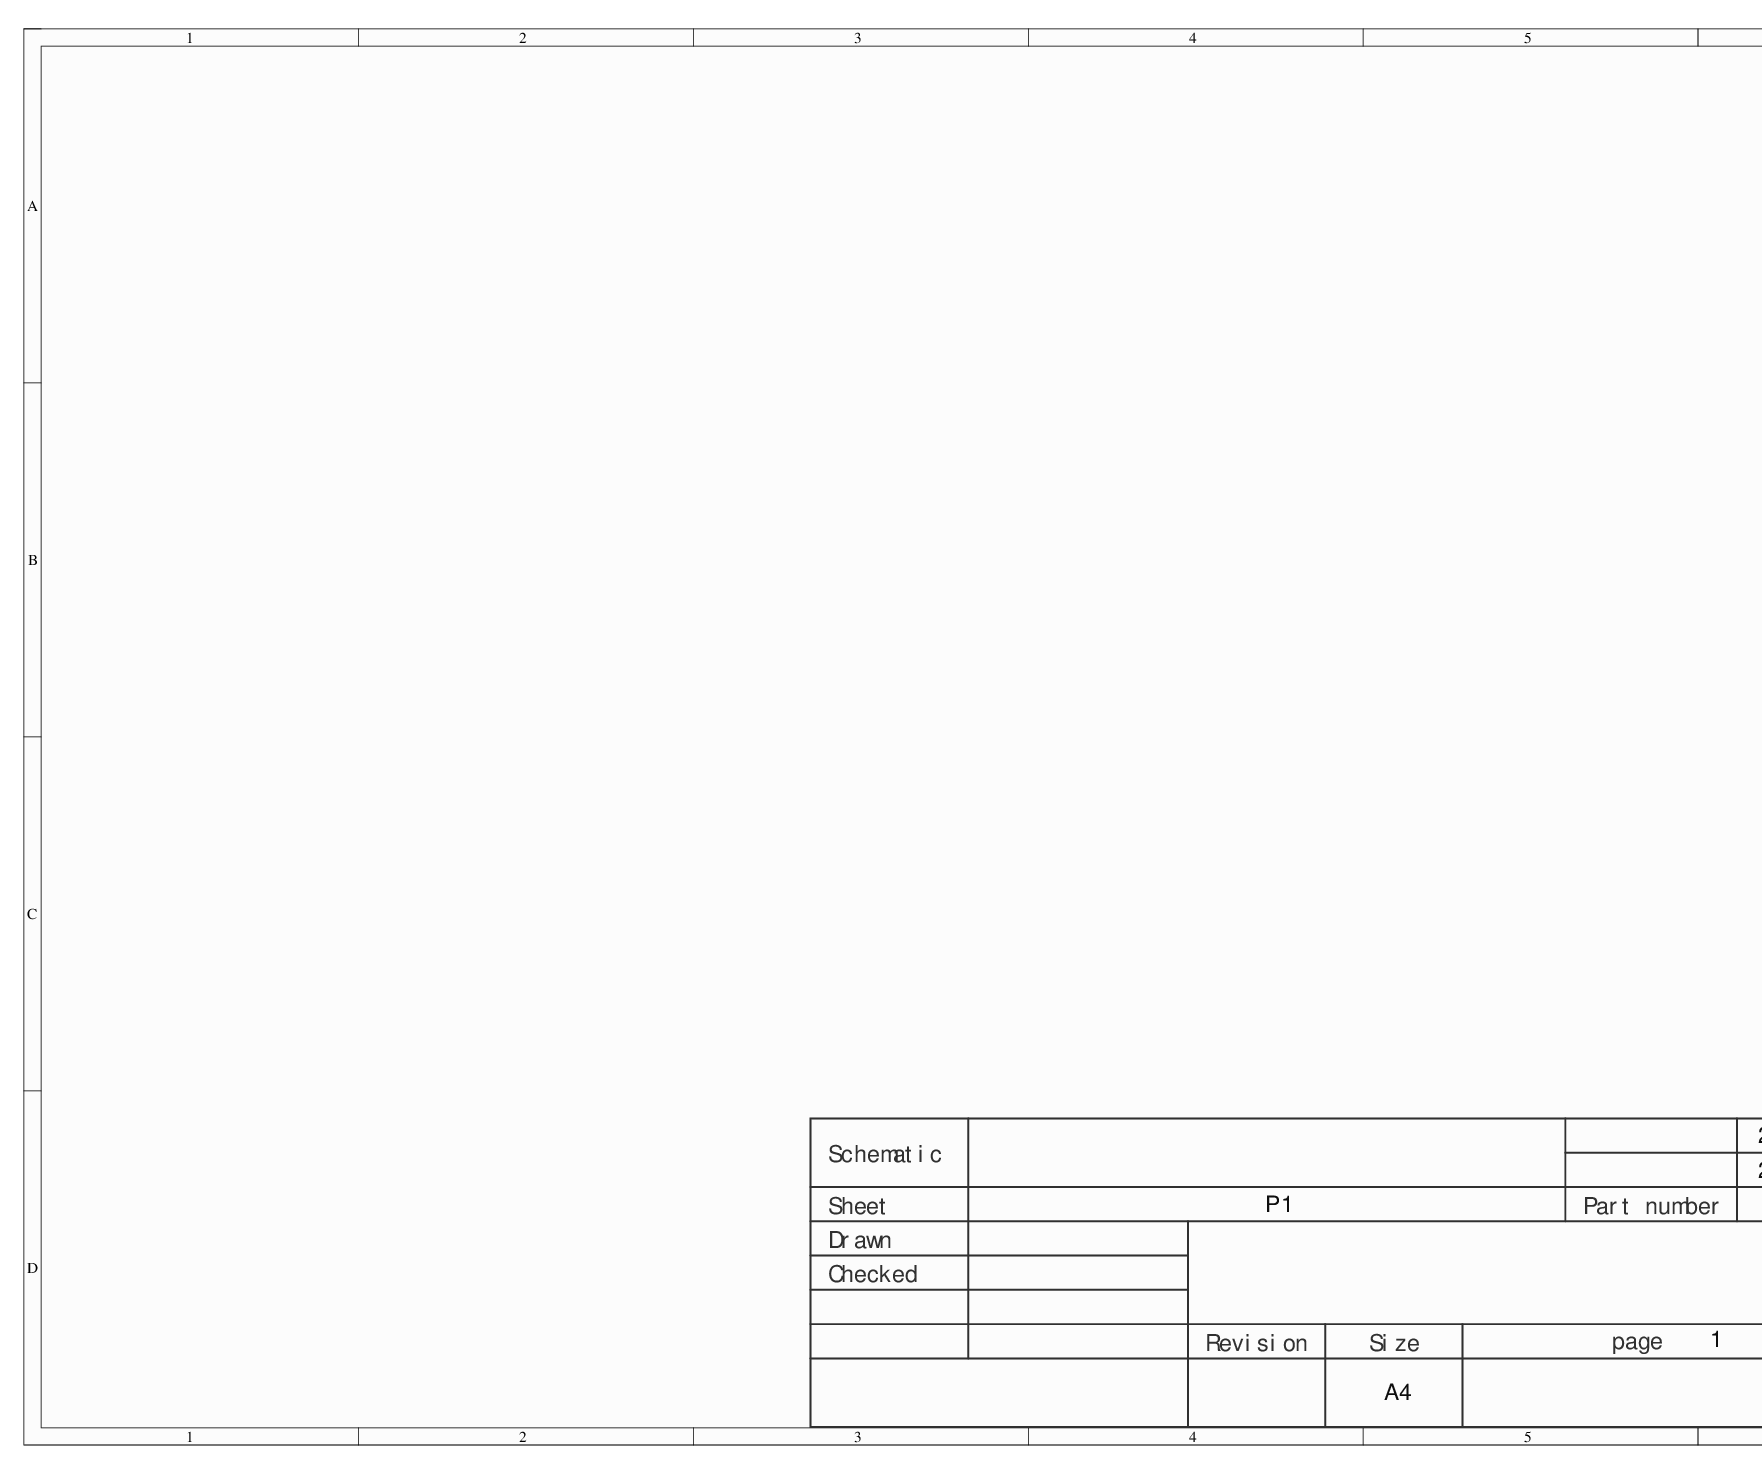
[diagram p0: MISC82093-2.schdoc, top left]
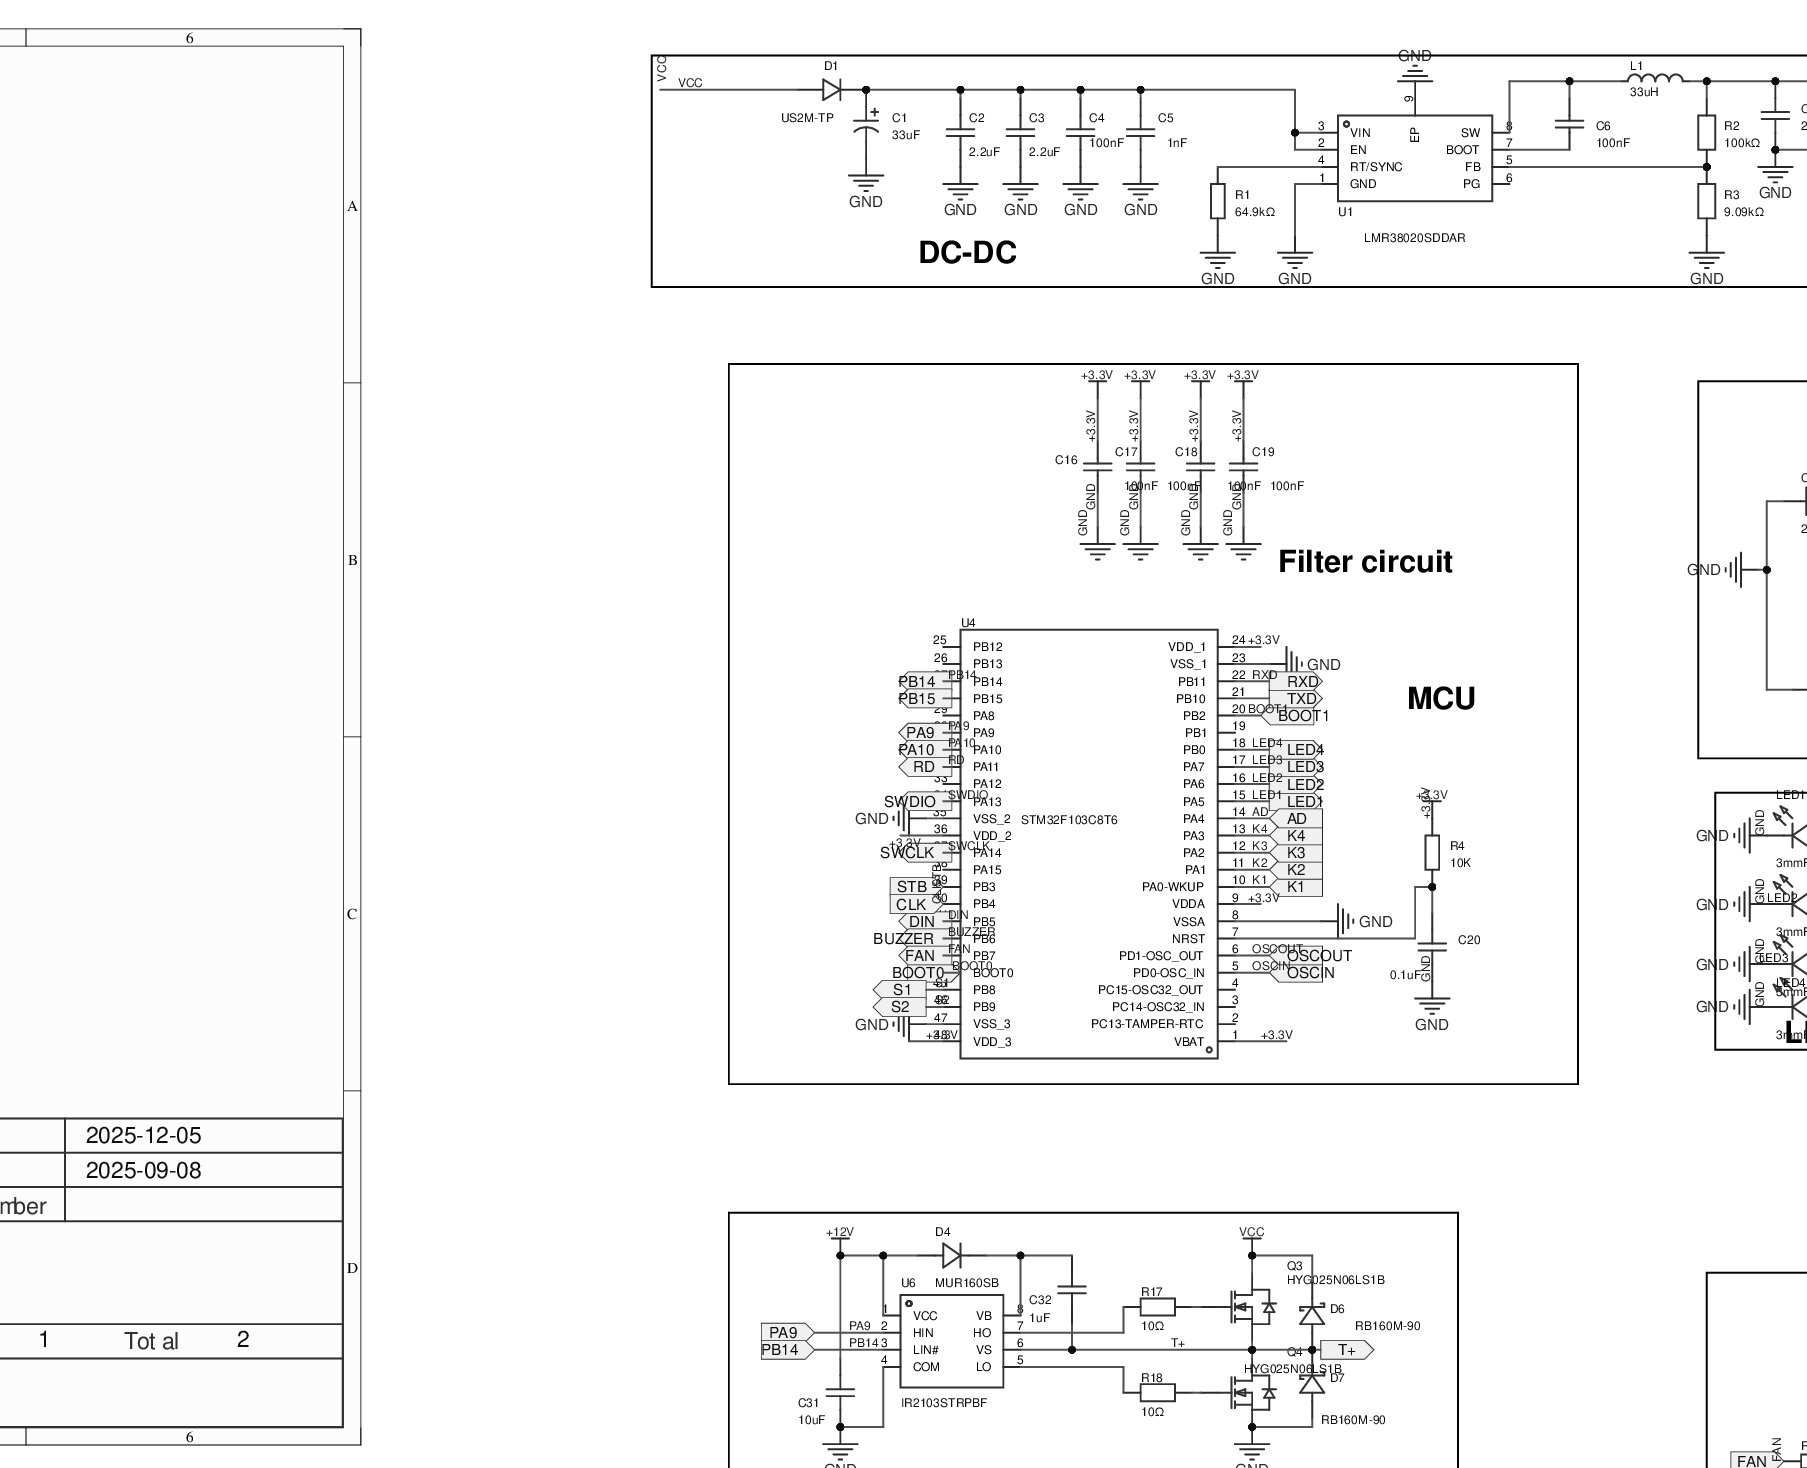
[diagram p1: MISC82093-2.schdoc, top middle]
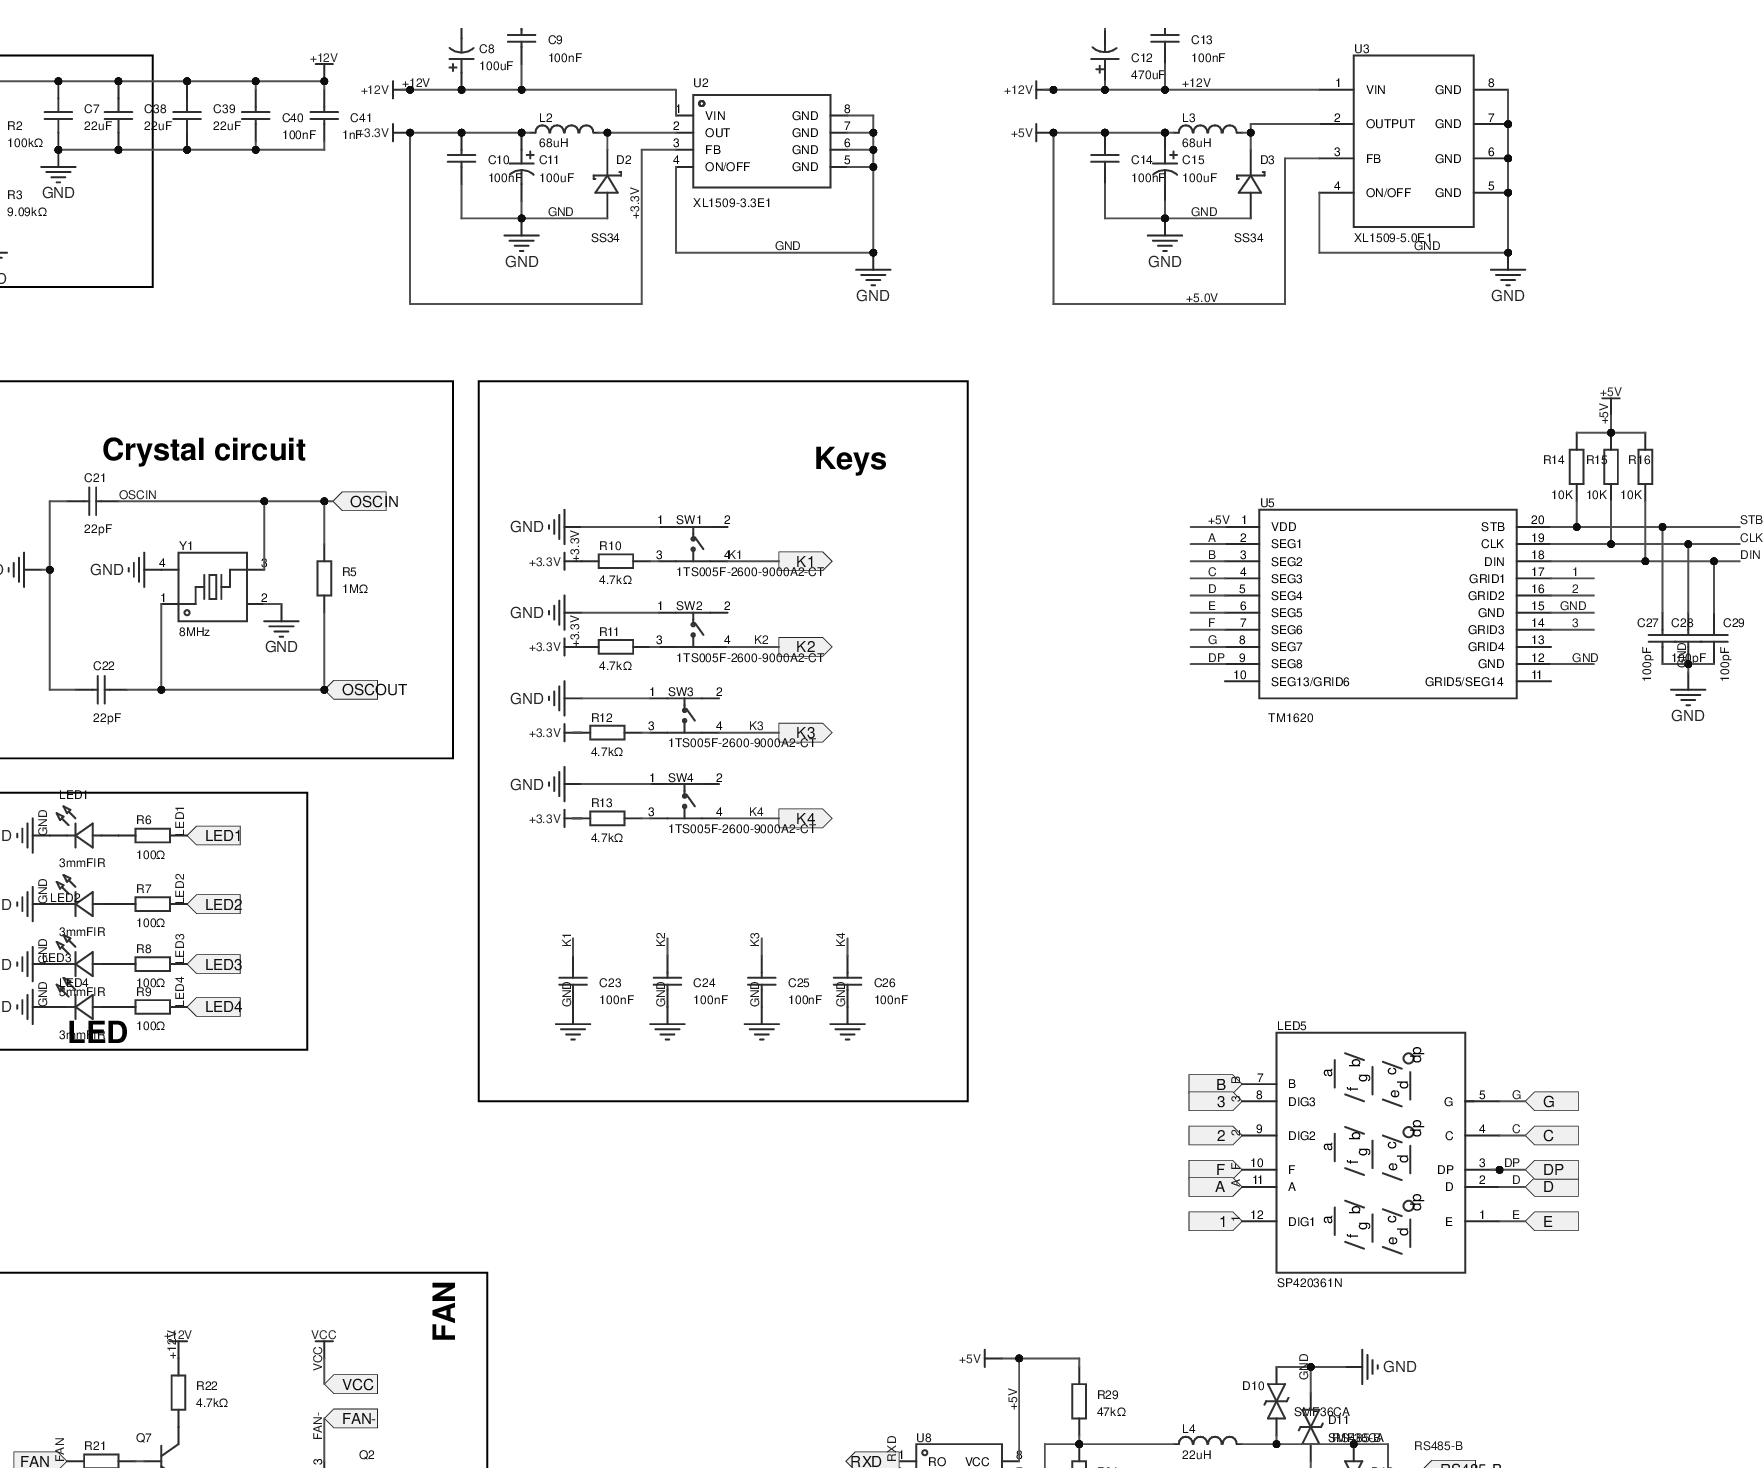
[diagram p2: MISC82093-2.schdoc, top right]
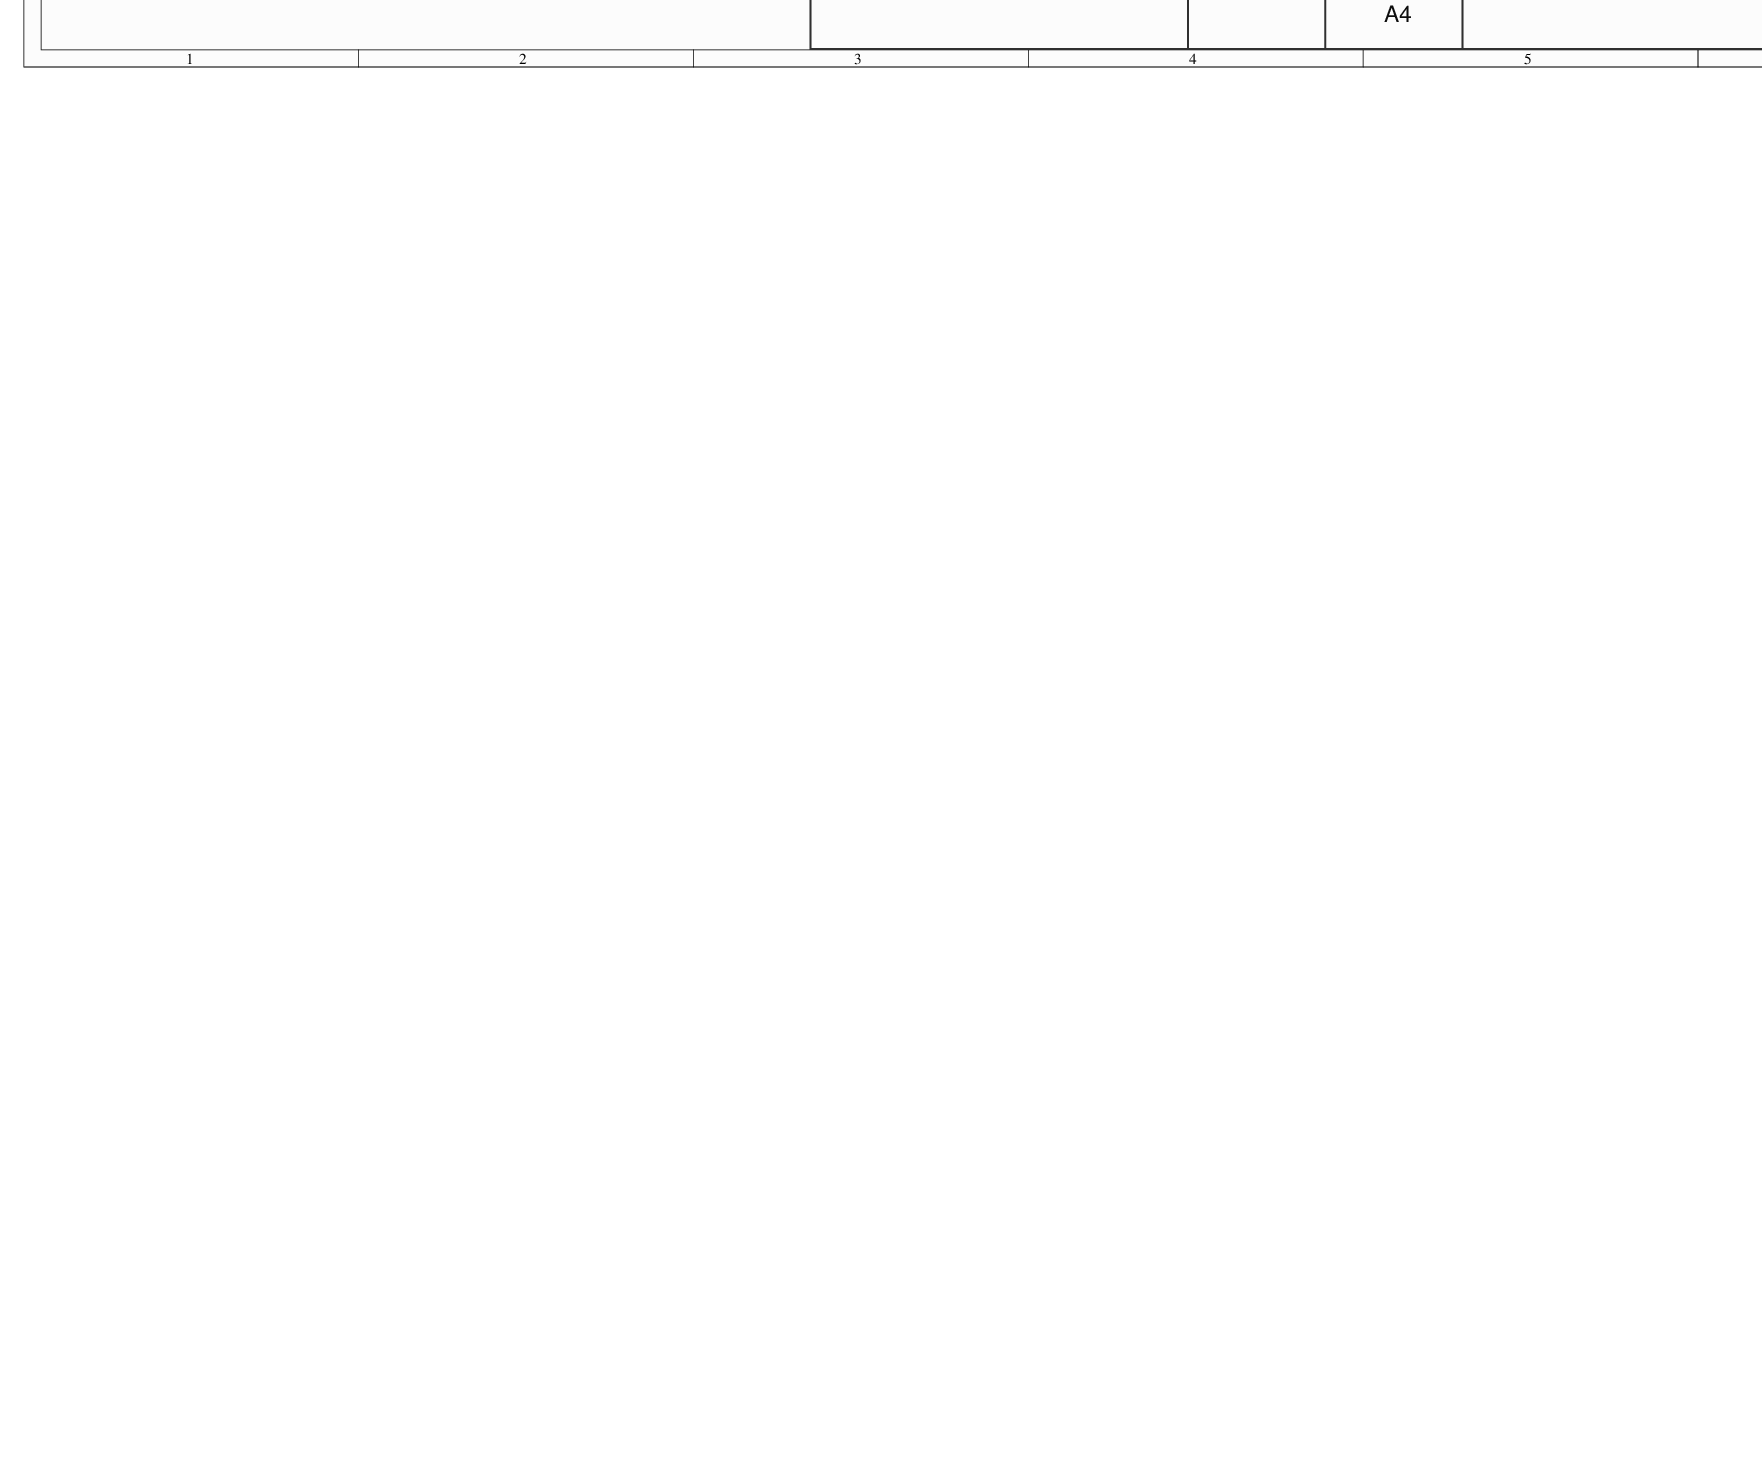
[diagram p3: MISC82093-2.schdoc, bottom left]
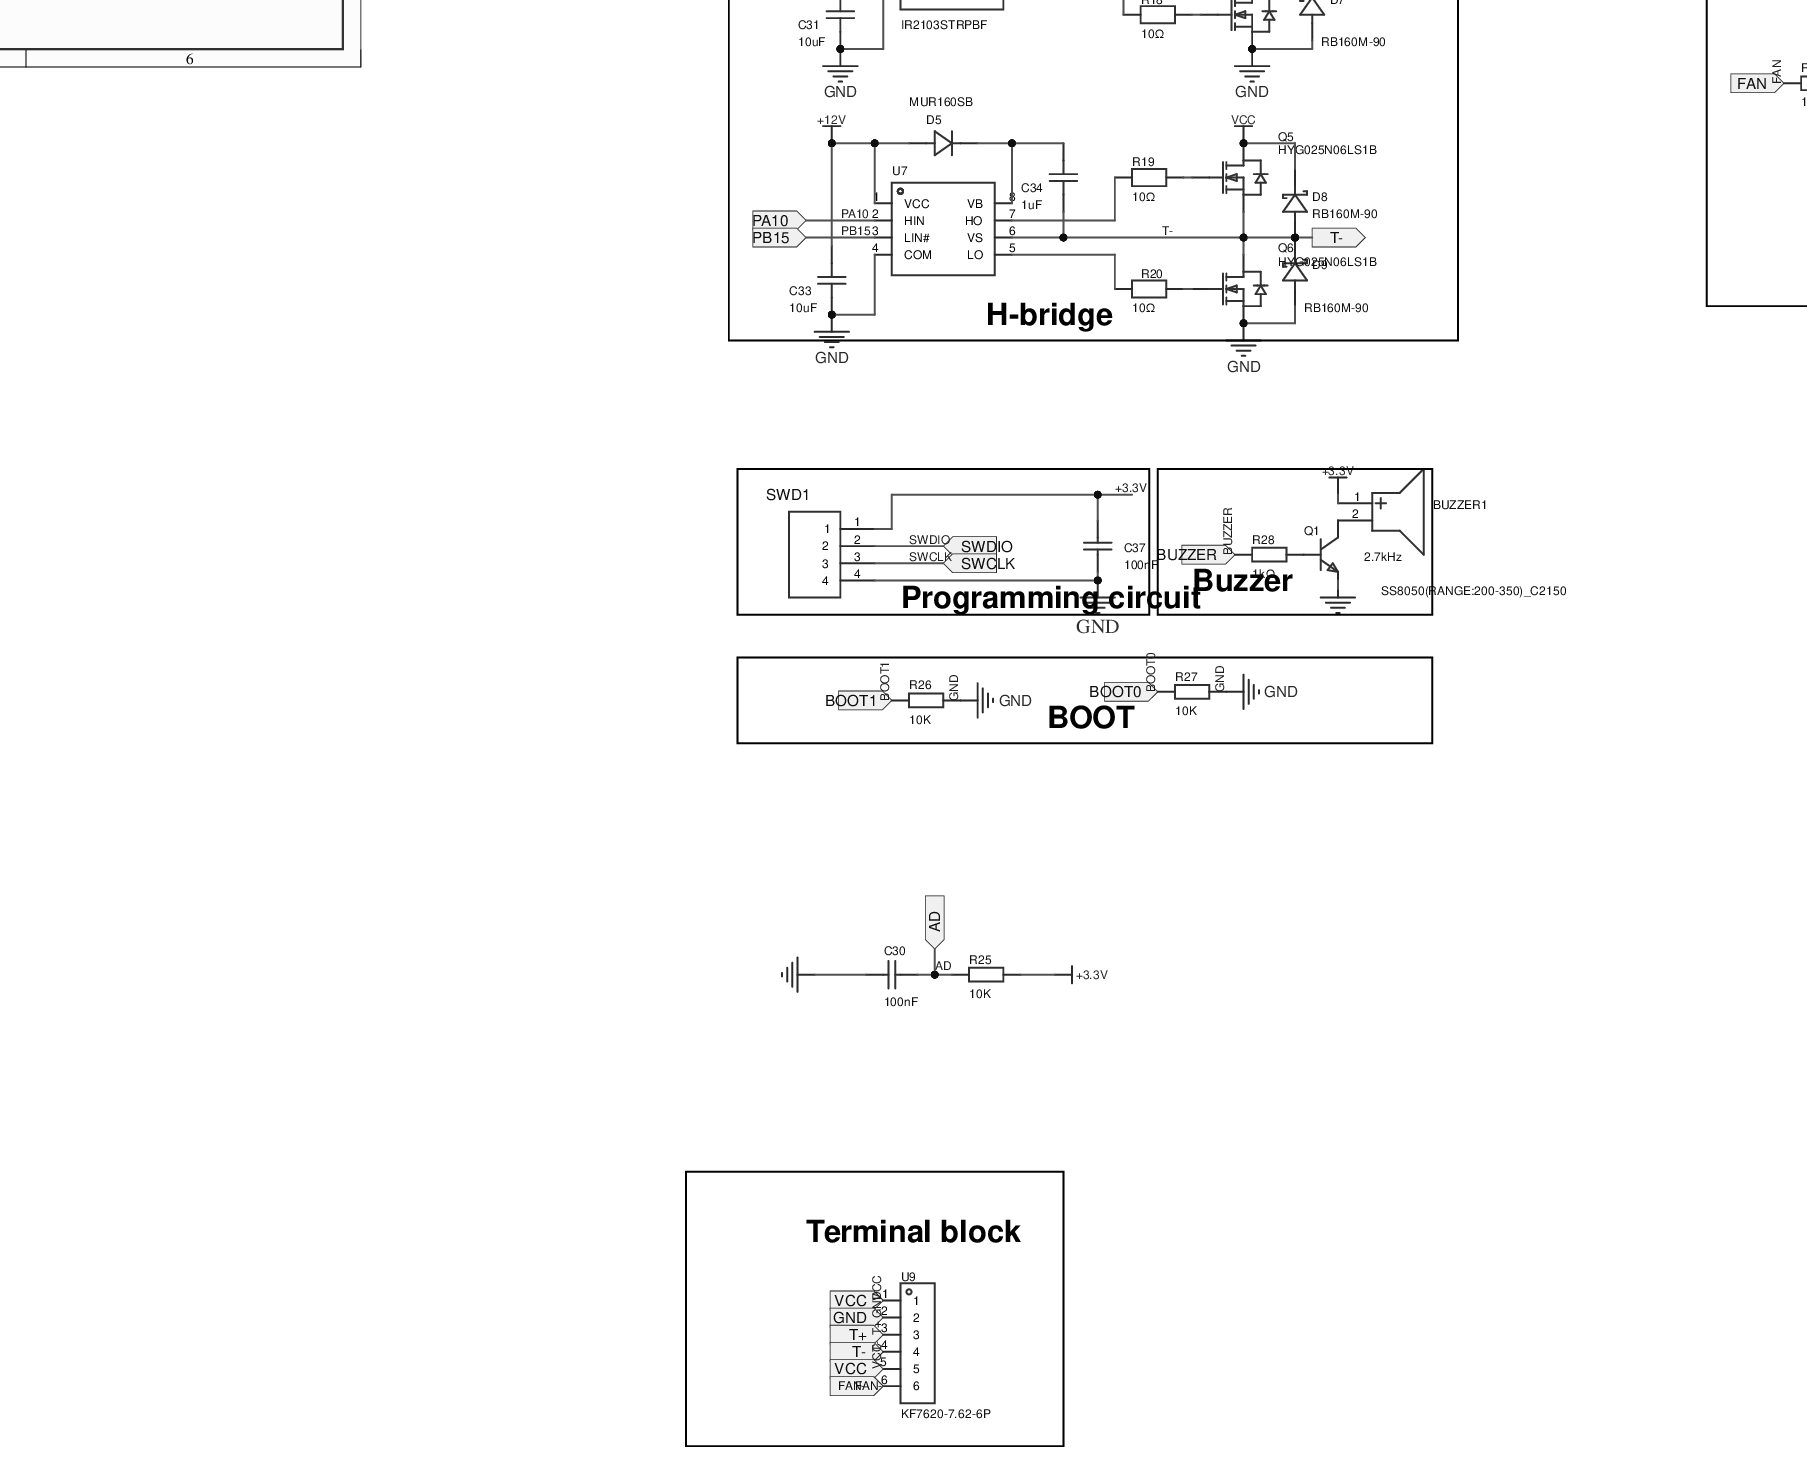
[diagram p4: MISC82093-2.schdoc, bottom middle]
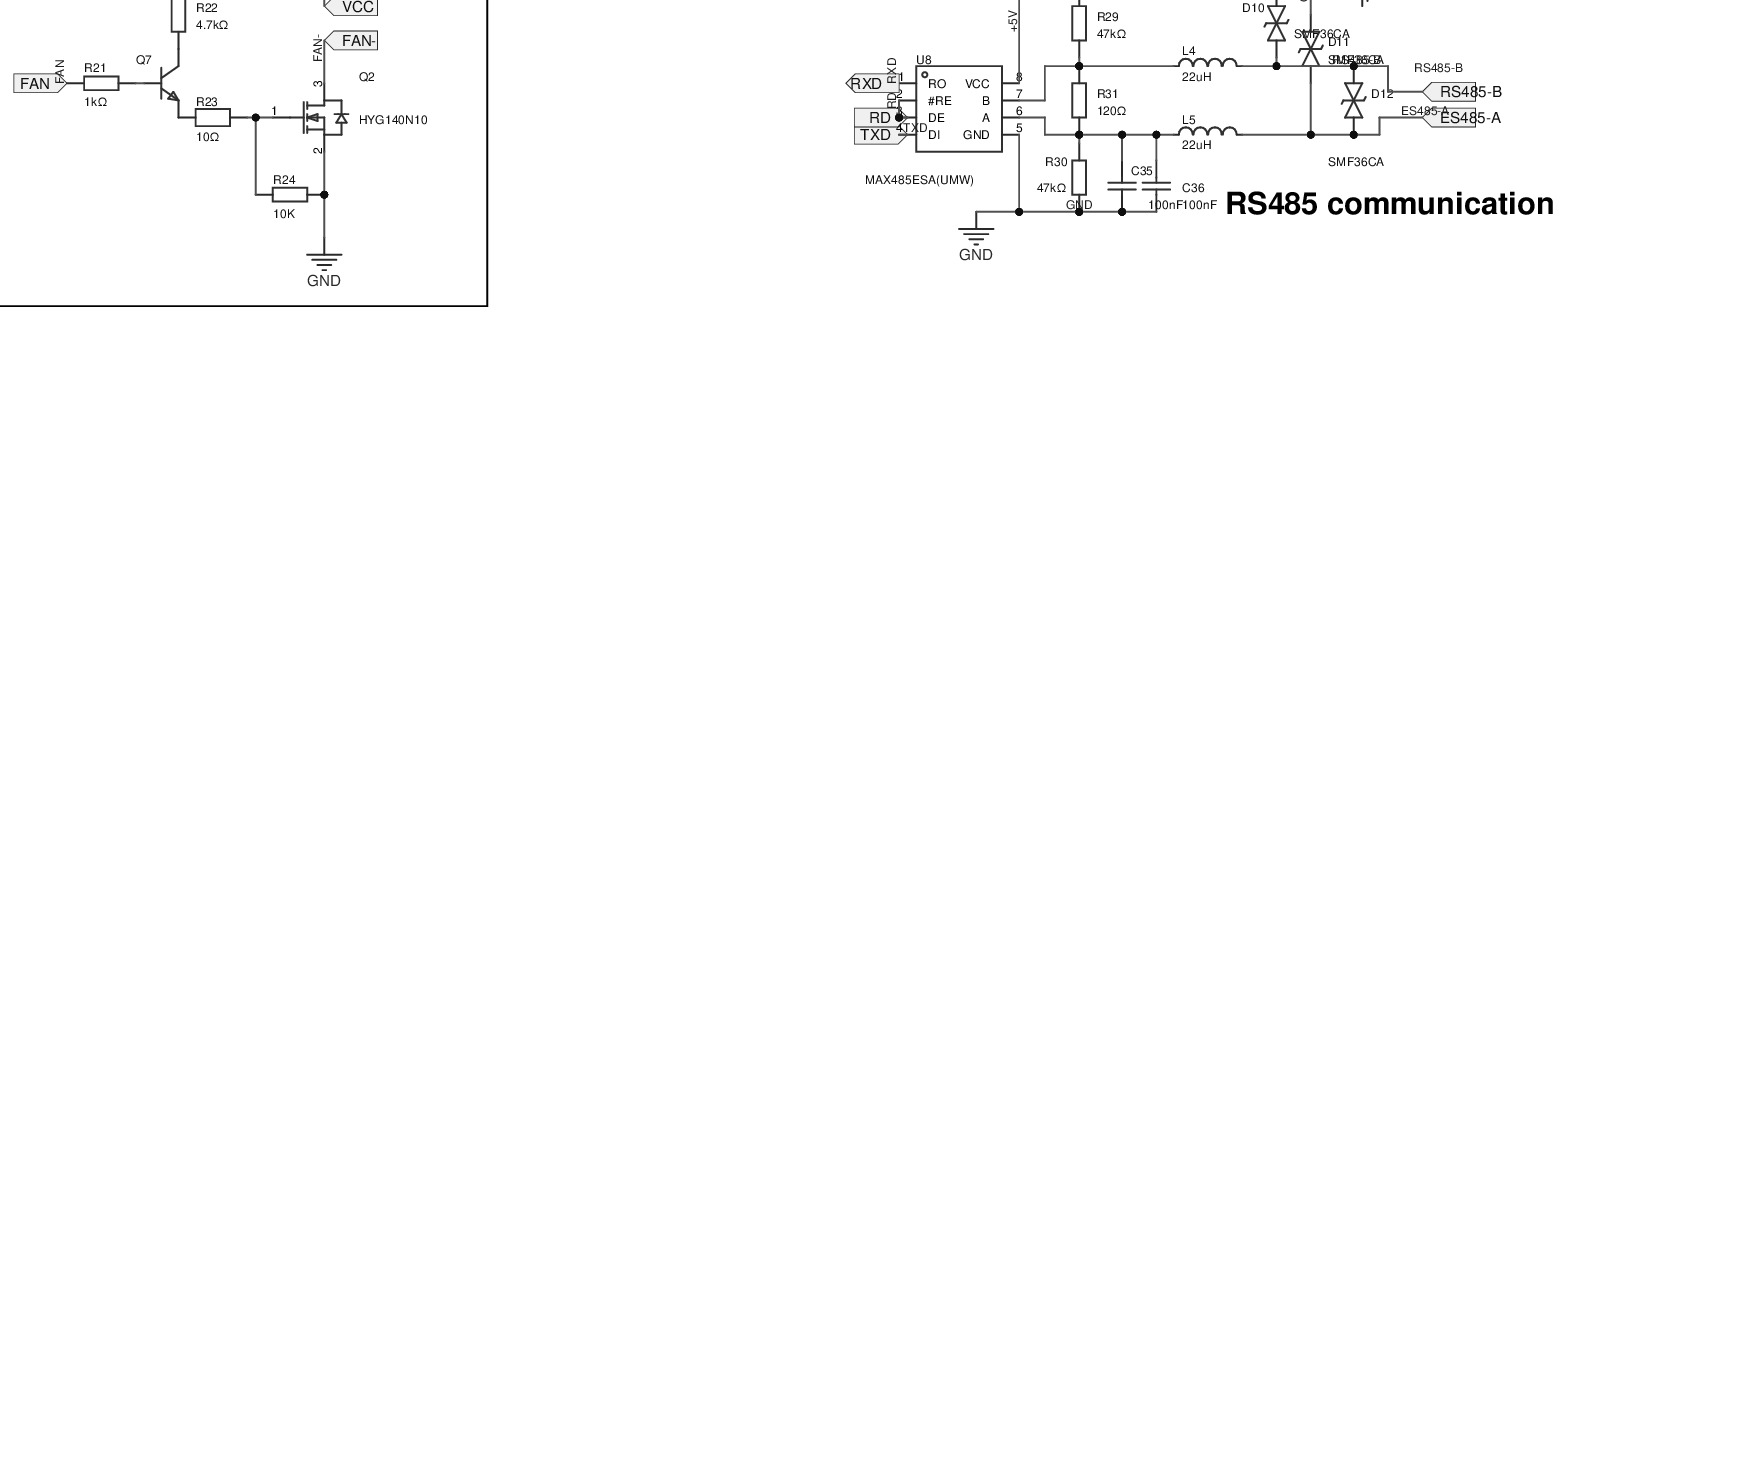
[diagram p5: MISC82093-2.schdoc, bottom right]
# Altium schematic sheet MISC82093-2.schdoc (part 1 of 2)
size 297 x 209 mm; Version: V1.0; @Project Name: MISC82093; @Page Count: 2; @Update Date: 2025-12-05; @Create Date: 2025-09-08; @Schematic Name: MISC82093; @Page No: 1; @Board Name: MISC82093; @Create Time: 16:21:40; @Update Time: 16:58:32

## Parts
BUZZER1  2.7kHz  [BUZ-SMD_L9.6-W9.6-LS10.0-R]
C1  33uF  [CAP-TH_BD8.0-P3.50-D1.0-FD]
C2  2.2uF  [C1206]
C3  2.2uF  [C1206]
C4  100nF  [C1206]
C5  1nF  [C1206]
C6  100nF  [C0805]
C7  22uF  [C1210]
C8  100uF  [CAP-SMD_BD6.3-L6.6-W6.6-LS7.3-FD_JVS25V100M6X4]
C9  100nF  [C0805]
C10  100nF  [C0805]
C11  100uF  [CAP-SMD_BD6.3-L6.6-W6.6-LS7.3-FD_JVS25V100M6X4]
C12  470uF  [CAP-TH_BD10.0-P5.00-D1.0-FD]
C13  100nF  [C0805]
C14  100nF  [C0805]
C15  100uF  [CAP-SMD_BD6.3-L6.6-W6.6-LS7.3-FD_JVS25V100M6X4]
C16  100nF  [C0805]
C17  100nF  [C0805]
C18  100nF  [C0805]
C19  100nF  [C0805]
C20  0.1uF  [C0805]
C21  22pF  [C0805]
C22  22pF  [C0805]
C23  100nF  [C0805]
C24  100nF  [C0805]
C25  100nF  [C0805]
C26  100nF  [C0805]
C27  100pF  [C0805]
C28  100pF  [C0805]
C29  100pF  [C0805]
C30  100nF  [C0805]
C31  10uF  [C0805]
C32  1uF  [C0805]
C33  10uF  [C0805]
C34  1uF  [C0805]
C35  100nF  [C0805]
C36  100nF  [C0805]
C37  100nF  [C0805]
C38  22uF  [C1210]
C39  22uF  [C1210]
C40  100nF  [C0805]
C41  1nF  [C0805]
D1  US2M-TP  [SMB_L4.6-W3.6-LS5.3-RD]
D2  SS34  [SMA_L4.3-W2.6-LS5.2-RD]
D3  SS34  [SMA_L4.3-W2.6-LS5.2-RD]
D4  MUR160SB  [SMB_L4.6-W3.6-LS5.3-RD]
D5  MUR160SB  [SMB_L4.6-W3.6-LS5.3-RD]
D6  RB160M-90  [SOD-123FL_L2.7-W1.8-LS3.7-RD]
D7  RB160M-90  [SOD-123FL_L2.7-W1.8-LS3.7-RD]
D8  RB160M-90  [SOD-123FL_L2.7-W1.8-LS3.7-RD]
D9  RB160M-90  [SOD-123FL_L2.7-W1.8-LS3.7-RD]
D10  SMF36CA  [SOD-123_L2.7-W1.8-LS3.7-BI]
D11  SMF36CA  [SOD-123_L2.7-W1.8-LS3.7-BI]
D12  SMF36CA  [SOD-123_L2.7-W1.8-LS3.7-BI]
L1  33uH  [IND-SMD_L11.5-W10.0_FXL1040]
L2  68uH  [IND-SMD_L7.1-W6.6_H5.0]
L3  68uH  [IND-SMD_L7.1-W6.6_H5.0]
L4  22uH  [L1206]
L5  22uH  [L1206]
LED1  3mmFIR  [LED-TH_BD3.0-P2.54-FD]
LED2  3mmFIR  [LED-TH_BD3.0-P2.54-FD]
LED3  3mmFIR  [LED-TH_BD3.0-P2.54-FD]
LED4  3mmFIR  [LED-TH_BD3.0-P2.54-FD]
LED5  SP420361N  [LED-SEG-TH_SP420361N]
Q1  SS8050(RANGE:200-350)  [SOT-23-3_L2.9-W1.3-P1.90-LS2.4-BR]  (value not drawn)
Q2  HYG140N10  [TO-252-3_L6.6-W6.1-P4.58-LS10.1-BR]
Q3  HYG025N06LS1B  [TO-263-2_L10.2-W8.7-P5.08-LS15.1-BR]
Q4  HYG025N06LS1B  [TO-263-2_L10.2-W8.7-P5.08-LS15.1-BR]
Q5  HYG025N06LS1B  [TO-263-2_L10.2-W8.7-P5.08-LS15.1-BR]
Q6  HYG025N06LS1B  [TO-263-2_L10.2-W8.7-P5.08-LS15.1-BR]
Q7  SS8050(RANGE:200-350)  [SOT-23-3_L2.9-W1.3-P1.90-LS2.4-BR]  (value not drawn)
R1  64.9kΩ  [R0805]
R2  100kΩ  [R0805]
R3  9.09kΩ  [R0805]
R4  10K  [R0805]
R5  1MΩ  [R0805]
R6  100Ω  [R0805]
R7  100Ω  [R0805]
R8  100Ω  [R0805]
R9  100Ω  [R0805]
R10  4.7kΩ  [R0805]
R11  4.7kΩ  [R0805]
R12  4.7kΩ  [R0805]
R13  4.7kΩ  [R0805]
R14  10K  [R0805]
R15  10K  [R0805]
R16  10K  [R0805]
R17  10Ω  [R0805]
R18  10Ω  [R0805]
R19  10Ω  [R0805]
R20  10Ω  [R0805]
R21  1kΩ  [R0805]
R22  4.7kΩ  [R0805]
R23  10Ω  [R0805]
R24  10K  [R0805]
R25  10K  [R0805]
R26  10K  [R0805]
R27  10K  [R0805]
R28  1kΩ  [R0805]
R29  47kΩ  [R0805]
R30  47kΩ  [R0805]
R31  120Ω  [R0805]
SW1  1TS005F-2600-9000A2-CT  [SW-SMD_4P-L6.0-W6.0-P4.50-LS9.0-2]
SW2  1TS005F-2600-9000A2-CT  [SW-SMD_4P-L6.0-W6.0-P4.50-LS9.0-2]
SW3  1TS005F-2600-9000A2-CT  [SW-SMD_4P-L6.0-W6.0-P4.50-LS9.0-2]
SW4  1TS005F-2600-9000A2-CT  [SW-SMD_4P-L6.0-W6.0-P4.50-LS9.0-2]
SWD1  220S-1*4P H=8.5MM Ytype Gold-plated  [DIP-1X4P2.54]  (value not drawn)
U1  LMR38020SDDAR  [ESOP-8_L4.9-W3.9-P1.27-LS6.0-BL-EP-1]
U2  XL1509-3.3E1  [SOP-8_L4.9-W3.9-P1.27-LS6.0-BL]
U3  XL1509-5.0E1  [SOIC-8_L5.0-W4.0-P1.27-LS6.0-BL]
U4  STM32F103C8T6  [LQFP-48_L7.0-W7.0-P0.50-LS9.0-BL]
U5  TM1620  [SOIC-20_L13.0-W7.6-P1.27-LS10.3-BL]
U6  IR2103STRPBF  [SOIC-8_L4.9-W3.9-P1.27-LS6.0-BL]
U7  (no value)  [SOIC-8_L4.9-W3.9-P1.27-LS6.0-BL]
U8  MAX485ESA(UMW)  [SOP-8_L5.0-W4.0-P1.27-LS6.0-BL]
U9  KF7620-7.62-6P  [CONN-TH_6P-P7.62_KF7620-7.62-6P]
Y1  8MHz  [CRYSTAL-SMD_4P-L3.2-W2.5-BL]

## Blocks framed on the sheet
DC-DC: C1-C7 C38 D1 L1 R1-R3 U1
Crystal circuit: C21 C22 R5 Y1
Keys: C23-C26 R10-R13 SW1-SW4
LED: LED1-LED4 R6-R9
H-bridge: C31-C34 D4-D9 Q3-Q6 R17-R20 U6 U7
FAN: Q2 Q7 R21-R24
Programming circuit: C37 SWD1
Buzzer: BUZZER1 Q1 R28
BOOT: R26 R27
Terminal block: U9

## Ports
1 (in), 2 (in), 3 (in), A (in), AD (in), B (in), BOOT0 (in), BOOT1 (in), BUZZER (in), BUZZER (out), C (in), CLK (in), D (in), DIN (out), DP (in), E (in), ES485-A (in), F (in), FAN (in), FAN (out), FAN- (in), G (in), GND (in), K1 (in), K1 (out), K2 (in), K2 (out), K3 (in), K3 (out), K4 (in), K4 (out), LED1 (in), LED1 (out), LED2 (in), LED2 (out), LED3 (in), LED3 (out), LED4 (in), LED4 (out), OSCIN (in), OSCOUT (in), PA9 (in), PA9 (out), PA10 (in), PA10 (out), PB14 (in), PB14 (out), PB15 (in), PB15 (out), RD (in), RD (out), RS485-B (in), RXD (out), S1 (out), S2 (out), STB (in), SWCLK (in), SWCLK (out), SWDIO (in), SWDIO (out), T+ (in), T+ (out), T- (in), T- (out), TXD (in), TXD (out), VCC (in)

## Nets
+3.3V: BUZZER1.1(+) C10.2 C11.1 C16.2 C17.2 C18.2 C19.2 C37.2 L2.1 R4.2 R10.1 R11.1 R12.1 R13.1 R25.2 SWD1.1 U2.3(FB) U4.1(VBAT) U4.9(VDDA) U4.24(VDD_1) U4.36(VDD_2) U4.48(VDD_3)
+5.0V: C14.2 C15.1 L3.1 R14.2 R15.2 R16.2 R29.2 U3.3(FB) U5.1(VDD) U8.8(VCC)  [also labelled +5V]
+12V: C7.2 C8.1 C9.1 C12.1 C13.1 C31.2 C33.2 C38.2 C39.2 C40.2 C41.2 D4.2(A) D5.2(A) L1.2 R2.2 R22.2 U2.1(VIN) U3.1(VIN) U6.1(VCC) U7.1(VCC)
GND: C1.2 C2.1 C3.1 C4.1 C5.1 C7.1 C8.2 C9.2 C10.1 C11.2 C12.2 C13.2 C14.1 C15.2 C16.1 C17.1 C18.1 C19.1 C20.1 C21.2 C22.2 C23.1 C24.1 C25.1 C26.1 C27.2 C28.2 C29.1 C30.2 C31.1 C33.1 C35.1 C36.2 C37.1 C38.1 C39.1 C40.1 C41.1 D2.2(A) D3.2(A) D7.2(+) D9.2(+) D10.2 D11.2 LED1.2(K) LED2.2(K) LED3.2(K) LED4.2(K) Q1.2(E) Q2.2(S) Q4.3(S) Q6.3(S) R1.1 R3.1 R24.2 R26.2 R27.2 R30.1 SW1.1 SW2.1 SW3.1 SW4.1 SWD1.4 U1.1(GND) U1.9(EP) U2.4(ON/OFF) U2.5(GND) U2.6(GND) U2.7(GND) U2.8(GND) U3.4(ON/OFF) U3.5(GND) U3.6(GND) U3.7(GND) U3.8(GND) U4.8(VSSA) U4.23(VSS_1) U4.35(VSS_2) U4.47(VSS_3) U5.12(GND) U5.15(GND) U6.4(COM) U7.4(COM) U8.5(GND) U9.2 Y1.2(GND) Y1.4(GND) ; port GND
VCC: D1.2(A) D6.1(-) D8.1(-) Q3.4(D) Q5.4(D) U9.1 U9.5 ; port VCC
1: LED5.12(DIG1) U5.17(GRID1) ; port 1
2: LED5.9(DIG2) U5.16(GRID2) ; port 2
3: LED5.8(DIG3) U5.14(GRID3) ; port 3
A: LED5.11(A) U5.2(SEG1) ; port A
AD: C30.1 R25.1 U4.14(PA4) ; port AD
B: LED5.7(B) U5.3(SEG2) ; port B
BOOT0: R27.1 U4.44(BOOT0) ; port BOOT0
BOOT1: R26.1 U4.20(PB2) ; port BOOT1
BUZZER: R28.1 U4.42(PB6) ; port BUZZER
C: LED5.4(C) U5.4(SEG3) ; port C
CLK: C28.1 R15.1 U4.40(PB4) U5.19(CLK) ; port CLK
D: LED5.2(D) U5.5(SEG4) ; port D
DIN: C29.2 R16.1 U4.41(PB5) U5.18(DIN) ; port DIN
DP: LED5.3(DP) U5.9(SEG8) ; port DP
E: LED5.1(E) U5.6(SEG5) ; port E
ES485-A: D11.1 D12.1 L5.2 ; port ES485-A
F: LED5.10(F) U5.7(SEG6) ; port F
FAN: R21.1 U4.43(PB7) ; port FAN
FAN-: Q2.3(D) U9.6 ; port FAN-
G: LED5.5(G) U5.8(SEG7) ; port G
K1: C23.2 SW1.4 U4.10(PA0-WKUP) ; port K1
K2: C24.2 SW2.4 U4.11(PA1) ; port K2
K3: C25.2 SW3.4 U4.12(PA2) ; port K3
K4: C26.2 SW4.4 U4.13(PA3) ; port K4
LED1: R6.2 U4.15(PA5) ; port LED1
LED2: R7.2 U4.16(PA6) ; port LED2
LED3: R8.2 U4.17(PA7) ; port LED3
LED4: R9.2 U4.18(PB0) ; port LED4
OSCIN: C21.1 R5.2 U4.5(PD0-OSC_IN) Y1.3 ; port OSCIN
OSCOUT: C22.1 R5.1 U4.6(PD1-OSC_OUT) Y1.1 ; port OSCOUT
PA9: U4.30(PA9) U6.2(HIN) ; port PA9
PA10: U4.31(PA10) U7.2(HIN) ; port PA10
PB14: U4.27(PB14) U6.3(LIN#) ; port PB14
PB15: U4.28(PB15) U7.3(LIN#) ; port PB15
RD: U4.32(PA11) U8.2(#RE) U8.3(DE) ; port RD
RS485-B: D10.1 D12.2 L4.2 ; port RS485-B
RXD: U4.22(PB11) U8.1(RO) ; port RXD
S1: U4.45(PB8) ; port S1
S2: U4.46(PB9) ; port S2
STB: C27.1 R14.1 U4.39(PB3) U5.20(STB) ; port STB
SWCLK: SWD1.3 U4.37(PA14) ; port SWCLK
SWDIO: SWD1.2 U4.34(PA13) ; port SWDIO
T+: C32.1 D6.2(+) D7.1(-) Q3.3(S) Q4.4(D) U6.6(VS) U9.3 ; port T+
T-: C34.1 D8.2(+) D9.1(-) Q5.3(S) Q6.4(D) U7.6(VS) U9.4 ; port T-
TXD: U4.21(PB10) U8.4(DI) ; port TXD
NetBUZZER1_2: BUZZER1.2(-) Q1.3(C)
NetC1_1: C1.1 C2.2 C3.2 C4.2 C5.2 D1.1(K) U1.2(EN) U1.3(VIN)
NetC6_1: C6.1 U1.7(BOOT)
NetC6_2: C6.2 L1.1 U1.8(SW)
NetC20_2: C20.2 R4.1 U4.7(NRST)
NetC32_2: C32.2 D4.1(K) U6.8(VB)
NetC34_2: C34.2 D5.1(K) U7.8(VB)
NetC35_2: C35.2 C36.1 L5.1 R30.2 R31.1 U8.6(A)
NetD2_1: D2.1(K) L2.2 U2.2(OUT)
NetD3_1: D3.1(K) L3.2 U3.2(OUTPUT)
NetL4_1: L4.1 R29.1 R31.2 U8.7(B)
NetLED1_1: LED1.1(A) R6.1
NetLED2_1: LED2.1(A) R7.1
NetLED3_1: LED3.1(A) R8.1
NetLED4_1: LED4.1(A) R9.1
NetQ1_1: Q1.1(B) R28.2
NetQ2_1: Q2.1(G) R23.2 R24.1
NetQ3_1: Q3.1(G) R17.2
NetQ4_1: Q4.1(G) R18.2
NetQ5_1: Q5.1(G) R19.2
NetQ6_1: Q6.1(G) R20.2
NetQ7_1: Q7.1(B) R21.2
NetQ7_2: Q7.2(E) R23.1
NetQ7_3: Q7.3(C) R22.1
NetR1_2: R1.2 U1.4(RT/SYNC)
NetR2_1: R2.1 R3.2 U1.5(FB)
NetR10_2: R10.2 SW1.3
NetR11_2: R11.2 SW2.3
NetR12_2: R12.2 SW3.3
NetR13_2: R13.2 SW4.3
NetR17_1: R17.1 U6.7(HO)
NetR18_1: R18.1 U6.5(LO)
NetR19_1: R19.1 U7.7(HO)
NetR20_1: R20.1 U7.5(LO)

Not connected (* = marked no-connect by the designer): SW1 2; SW2 2; SW3 2; SW4 2; U1 6(PG)*; U4 2(PC13-TAMPER-RTC)* 3(PC14-OSC32_IN)* 4(PC15-OSC32_OUT)* 19(PB1)* 25(PB12)* 26(PB13)* 29(PA8)* 33(PA12)* 38(PA15)*; U5 10(SEG13/GRID6)* 11(GRID5/SEG14)* 13(GRID4)*

## Notes on the sheet
- Filter circuit
- MCU
- RS485 communication
- Labels drawn without touching a wire or pin: GND, RS485-B, VCC
- 2025-12-05
- Schematic
- Sheet
- P1
- Part number
- 2025-09-08
- Checked
- Drawn
- Revision
- Size
- A4
- page
- 1
- Total
- 2